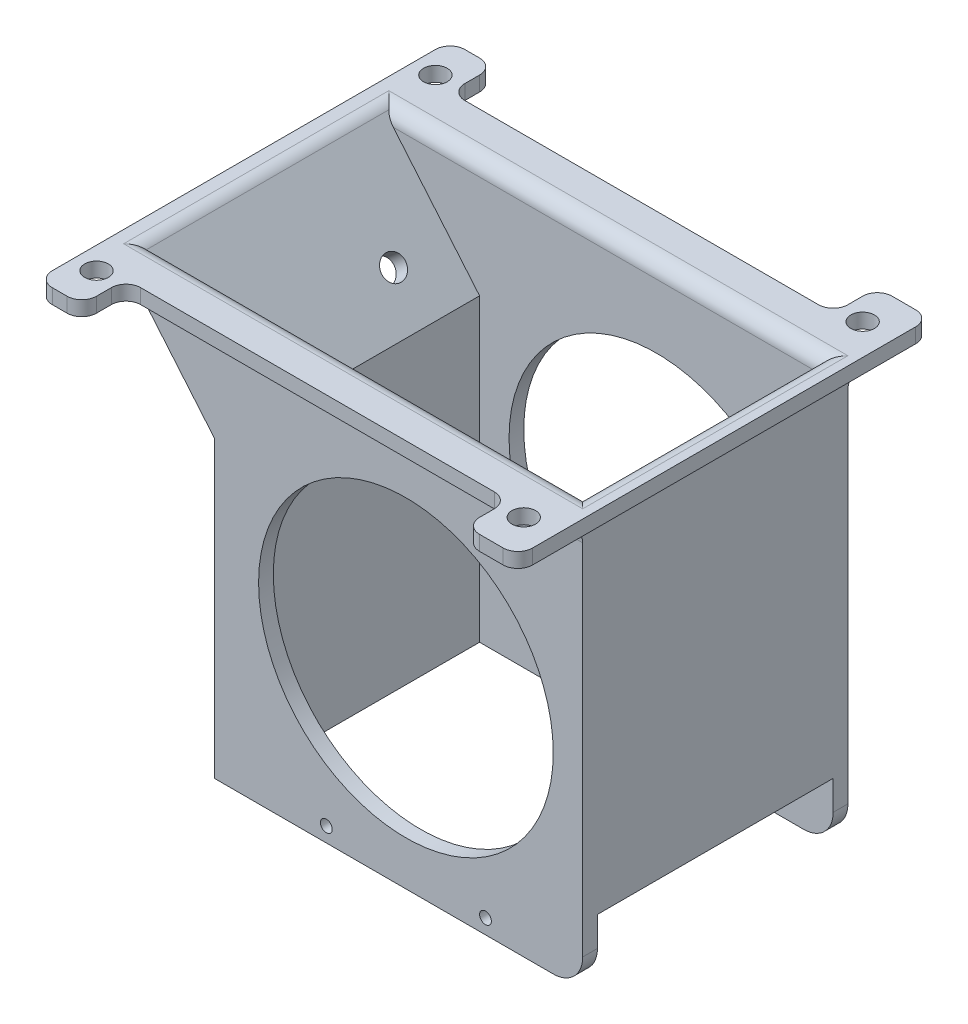
from build123d import *

# Parameters (mm, degrees)
EXTRUDE_1_DEPTH      = 45
SHELL_1_T            = -5
SKETCH_2_W           = 15
SKETCH_2_H           = 25
SKETCH_2_R           = 4
EXTRUDE_2_DEPTH      = 5
SKETCH_3_W           = 115
SKETCH_3_H           = 80
CUT_EXTRUDE_3_DEPTH  = 184.275749233
SKETCH_4_W           = 80
SKETCH_4_H           = 20
CUT_EXTRUDE_4_DEPTH  = 5
SKETCH_5_R           = 50
CUT_EXTRUDE_5_DEPTH  = 209.10361365
EXTRUDE_6_REACH      = 207.383
SKETCH_7_W           = 130
SKETCH_7_H           = 10
SKETCH_7_W_2         = 3
SKETCH_7_H_2         = 140
EXTRUDE_7_DEPTH      = 5
FILLET_1_R           = 5
FILLET_2_R           = 5
FILLET_3_R           = 5
FILLET_4_R           = 5
FILLET_5_R           = 5
FILLET_6_R           = 10
SKETCH_15_R          = 4
CUT_EXTRUDE_16_DEPTH = 187.54027319
SKETCH_16_R          = 2
CUT_EXTRUDE_17_DEPTH = 209.10361365


with BuildPart() as part:
    # 草图1 → 拉伸1 (new, symmetric)
    with BuildSketch(Plane.XY):
        Polygon((-65, 0), (60, 0), (60, 141.711375741), (-100, 141.711375741), (-65, 100), align=None)
    extrude(amount=EXTRUDE_1_DEPTH, both=True)

    # 抽壳1
    shell_1_openings = [part.faces().sort_by_distance(p)[0] for p in [
        (-20, 141.711375741, 0),
    ]]
    offset(amount=SHELL_1_T, openings=shell_1_openings, kind=Kind.INTERSECTION)

    # 草图2 → 拉伸2 (add)
    # profile 1 of 4: a face of its own
    with BuildSketch(Plane(origin=(0, 141.711375741, 0), x_dir=(1, 0, 0), z_dir=(0, 1, 0))):
        with Locations((52.5, 57.5)):
            Rectangle(SKETCH_2_W, SKETCH_2_H)
        with Locations(Location((52.5, 57.5, 0), (0, 0, 180))):
            Circle(SKETCH_2_R, mode=Mode.SUBTRACT)
    # profile 2 of 4: a face of its own
    with BuildSketch(Plane(origin=(0, 141.711375741, 0), x_dir=(1, 0, 0), z_dir=(0, 1, 0))):
        with Locations((-92.5, -57.5)):
            Rectangle(SKETCH_2_W, SKETCH_2_H)
        with Locations(Location((-92.5, -57.5, 0), (0, 0, 180))):
            Circle(SKETCH_2_R, mode=Mode.SUBTRACT)
    # profile 3 of 4: a face of its own
    with BuildSketch(Plane(origin=(0, 141.711375741, 0), x_dir=(1, 0, 0), z_dir=(0, 1, 0))):
        with Locations((52.5, -57.5)):
            Rectangle(SKETCH_2_W, SKETCH_2_H)
        with Locations((52.5, -57.5)):
            Circle(SKETCH_2_R, mode=Mode.SUBTRACT)
    # profile 4 of 4: a face of its own
    with BuildSketch(Plane(origin=(0, 141.711375741, 0), x_dir=(1, 0, 0), z_dir=(0, 1, 0))):
        with Locations((-92.5, 57.5)):
            Rectangle(SKETCH_2_W, SKETCH_2_H)
        with Locations((-92.5, 57.5)):
            Circle(SKETCH_2_R, mode=Mode.SUBTRACT)
    extrude(amount=-EXTRUDE_2_DEPTH)

    # 草图3 → 拉伸3 (cut, through all)
    with BuildSketch(Plane(origin=(0, 5, 0), x_dir=(1, 0, 0), z_dir=(0, 1, 0))):
        with Locations((-2.5, 0)):
            Rectangle(SKETCH_3_W, SKETCH_3_H)
    extrude(amount=-CUT_EXTRUDE_3_DEPTH, mode=Mode.SUBTRACT)

    # 草图4 → 拉伸4 (cut)
    with BuildSketch(Plane(origin=(60, 0, 0), x_dir=(0, 0, -1), z_dir=(1, 0, 0))):
        with Locations((0, 10)):
            Rectangle(SKETCH_4_W, SKETCH_4_H)
    extrude(amount=-CUT_EXTRUDE_4_DEPTH, mode=Mode.SUBTRACT)

    # 草图5 → 拉伸5 (cut, through all)
    with BuildSketch(Plane.XY.offset(45)):
        with Locations((0, 65)):
            Circle(SKETCH_5_R)
    extrude(amount=-CUT_EXTRUDE_5_DEPTH, mode=Mode.SUBTRACT)

    # 草图6 → 拉伸6 (add, up to next)
    with BuildSketch(Plane(origin=(0, 0, 40), x_dir=(-1, 0, 0), z_dir=(0, 0, -1)), mode=Mode.PRIVATE) as extrude_6_sk1:
        with BuildLine():
            Line((-55, 102.164254348), (-46.579364738, 88.116288209))
            ThreePointArc((-46.579364738, 88.116288209), (-51.147730221, 55.623983082), (-35.351205937, 26.864816261))
            Line((-35.351205937, 26.864816261), (-55, 26.864816261))
            Line((-55, 26.864816261), (-55, 102.164254348))
        make_face()
    extrude_6_tool1 = extrude(extrude_6_sk1.sketch, amount=EXTRUDE_6_REACH, mode=Mode.PRIVATE) - part.part
    add(extrude_6_tool1.solids().sort_by_distance((45.175603, 27.643024, 40))[0])

    # 草图7 → 拉伸7 (add)
    with BuildSketch(Plane(origin=(0, 141.711375741, 0), x_dir=(1, 0, 0), z_dir=(0, 1, 0))):
        with Locations((-20, 50)):
            Rectangle(SKETCH_7_W, SKETCH_7_H)
        with Locations((-20, -50)):
            Rectangle(SKETCH_7_W, SKETCH_7_H)
        with Locations((61.5, 0)):
            Rectangle(SKETCH_7_W_2, SKETCH_7_H_2)
    extrude(amount=-EXTRUDE_7_DEPTH)

    # 圆角1
    fillet_1_edges = [part.edges().sort_by_distance(p)[0] for p in [
        (-19.236481777, 141.711375741, -40),
        (-19.236481777, 141.711375741, 40),
    ]]
    fillet(fillet_1_edges, radius=FILLET_1_R)

    # 圆角2
    fillet_2_edges = [part.edges().sort_by_distance(p)[0] for p in [
        (55, 141.711375741, 0),
        (-93.472963553, 141.711375741, 0),
    ]]
    fillet(fillet_2_edges, radius=FILLET_2_R)

    # 圆角3
    fillet_3_edges = [part.edges().sort_by_distance(p)[0] for p in [
        (55, 102.164254348, 0),
    ]]
    fillet(fillet_3_edges, radius=FILLET_3_R)

    # 圆角4
    fillet_4_edges = [part.edges().sort_by_distance(p)[0] for p in [
        (45, 139.211375741, -55),
        (45, 139.211375741, -70),
        (63, 139.211375741, -70),
        (63, 139.211375741, 70),
        (45, 139.211375741, 55),
        (45, 139.211375741, 70),
        (-100, 139.211375741, -70),
        (-85, 139.211375741, -70),
        (-85, 139.211375741, -55),
        (-100, 139.211375741, 70),
        (-85, 139.211375741, 70),
        (-85, 139.211375741, 55),
    ]]
    fillet(fillet_4_edges, radius=FILLET_4_R)

    # 圆角5
    fillet_5_edges = [part.edges().sort_by_distance(p)[0] for p in [
        (-17.902250922, 136.711375741, -45),
        (-17.902250922, 136.711375741, 45),
    ]]
    fillet(fillet_5_edges, radius=FILLET_5_R)

    # 圆角6
    fillet_6_edges = [part.edges().sort_by_distance(p)[0] for p in [
        (60, 0, 42.5),
        (60, 0, -42.5),
    ]]
    fillet(fillet_6_edges, radius=FILLET_6_R)

    # 草图15 → 拉伸16 (cut, through all)
    with BuildSketch(Plane(origin=(14.927044092, 12.525277192, 0), x_dir=(0.6427876096865403, -0.7660444431189775, 0), z_dir=(0.7660444431189775, 0.6427876096865403, 0))):
        with Locations(Location((-132.835972882, -21.25, 0), (0, 0, 180))):
            Circle(SKETCH_15_R)
        with Locations(Location((-132.835972882, 21.25, 0), (0, 0, 180))):
            Circle(SKETCH_15_R)
    extrude(amount=-CUT_EXTRUDE_16_DEPTH, mode=Mode.SUBTRACT)

    # 草图16 → 拉伸17 (cut, through all)
    with BuildSketch(Plane.XY.offset(45)):
        with Locations((-27, 5)):
            Circle(SKETCH_16_R)
        with Locations((27, 5)):
            Circle(SKETCH_16_R)
    extrude(amount=-CUT_EXTRUDE_17_DEPTH, mode=Mode.SUBTRACT)


solid = part.part
